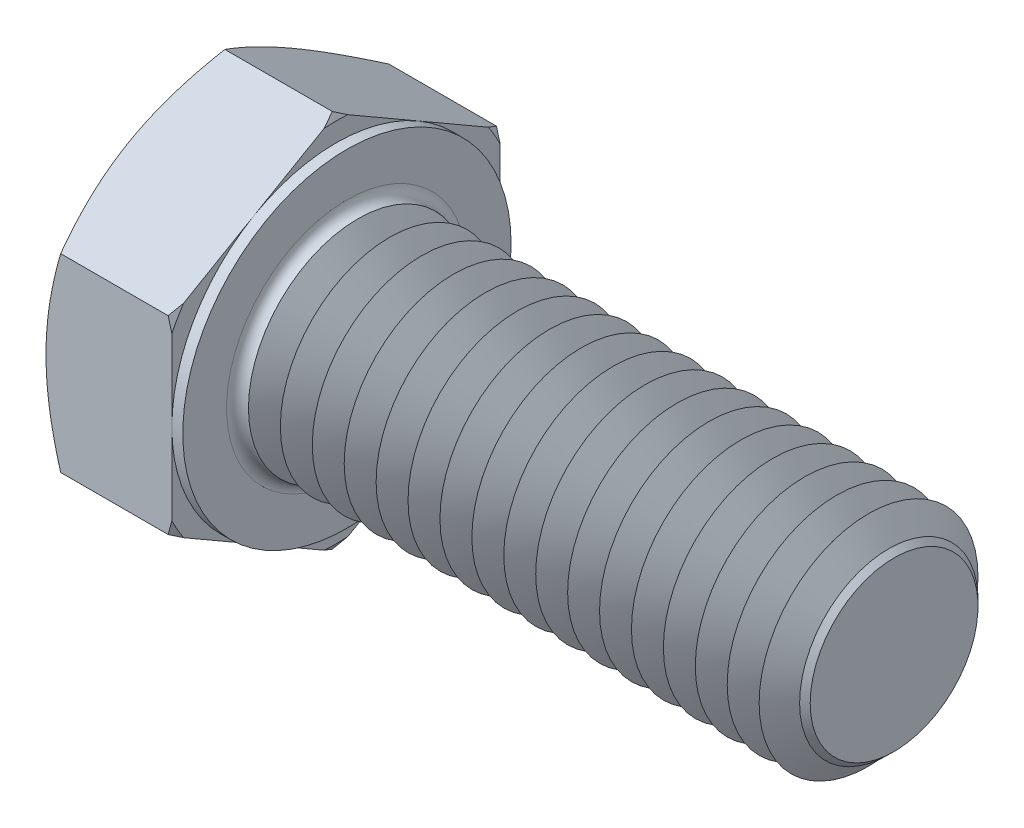
from build123d import *

# Parameters (mm, degrees)
EXTRUDE_374_DEPTH      = 7.5
SKETCH_4_W             = 0.6
SKETCH_4_H             = 11.392304845
CHAMFER_1914_SIZE      = 1.4
FILLET_1959_R          = 0.6
PATTERN_LINEAR_1_COUNT = 17
PATTERN_LINEAR_1_PITCH = 1.75


with BuildPart() as part:
    # 草图1 → Extrude 374 (new body)
    with BuildSketch(Plane(origin=(0, 0, 0), x_dir=(0, 0, -1), z_dir=(1, 0, 0))):
        Polygon((9, 5.196152423), (9, -5.196152423), (0, -10.392304845), (-9, -5.196152423), (-9, 5.196152423), (0, 10.392304845), align=None)
    extrude(amount=EXTRUDE_374_DEPTH)

    # 草图2 → 凸台-旋转1 (revolve)
    with BuildSketch(Plane.XY, mode=Mode.PRIVATE) as revolve_1_sk:
        Polygon((0, 0), (37.5, 0), (37.5, 4.4845), (37.5, 6), (0, 6), align=None)
    revolve(revolve_1_sk.sketch.rotate(Axis((0, 0, 0), (1, 0, 0)), 90), axis=Axis((0, 0, 0), (1, 0, 0)))

    # 草图3 → 切除-旋转1 (revolve, cut)
    with BuildSketch(Plane.XY):
        Polygon((0, 9), (3.690598923, 15.392304845), (3.690598923, 20.392304845), (-10, 20.392304845), (-10, 9), align=None)
    revolve(axis=Axis((0, 0, 0), (1, 0, 0)), mode=Mode.SUBTRACT)

    # 草图5 → 切除-旋转2 (revolve, cut)
    with BuildSketch(Plane.XY):
        Polygon((7.5, 9), (3.809401077, 15.392304845), (3.809401077, 20.392304845), (13.809401077, 20.392304845), (13.809401077, 9), align=None)
    revolve(axis=Axis((0, 0, 0), (1, 0, 0)), mode=Mode.SUBTRACT)

    # 草图4 → 切除-旋转3 (revolve, cut)
    with BuildSketch(Plane.XY, mode=Mode.PRIVATE) as cut_revolve_3_sk:
        with Locations((7.2, 14.696152423)):
            Rectangle(SKETCH_4_W, SKETCH_4_H)
    revolve(cut_revolve_3_sk.sketch.rotate(Axis((0, 0, 0), (1, 0, 0)), 270), axis=Axis((0, 0, 0), (1, 0, 0)), mode=Mode.SUBTRACT)

    # Chamfer 1914
    chamfer_1914_edges = [part.edges().sort_by_distance(p)[0] for p in [
        (37.5, 0, -6),
    ]]
    chamfer(chamfer_1914_edges, length=CHAMFER_1914_SIZE)

    # Fillet 1959
    fillet_1959_edges = [part.edges().sort_by_distance(p)[0] for p in [
        (7.5, 0, -6),
    ]]
    fillet(fillet_1959_edges, radius=FILLET_1959_R)

    # 草图6 → 切除-旋转4 (revolve, cut)
    with BuildSketch(Plane.XY):
        Polygon((8.974974333, -4.4845), (8.1, -6), (8.1, -7.5), (9.849948666, -7.5), (9.849948666, -6), align=None)
    cut_revolve_4 = revolve(axis=Axis((-3.175, 0, 0), (1, 0, 0)), mode=Mode.SUBTRACT)

    # 阵列(线性)1: 切除-旋转4 ×17
    with Locations(*[(i * PATTERN_LINEAR_1_PITCH, 0, 0) for i in range(1, PATTERN_LINEAR_1_COUNT)]):
        add(cut_revolve_4, mode=Mode.SUBTRACT)


solid = part.part
